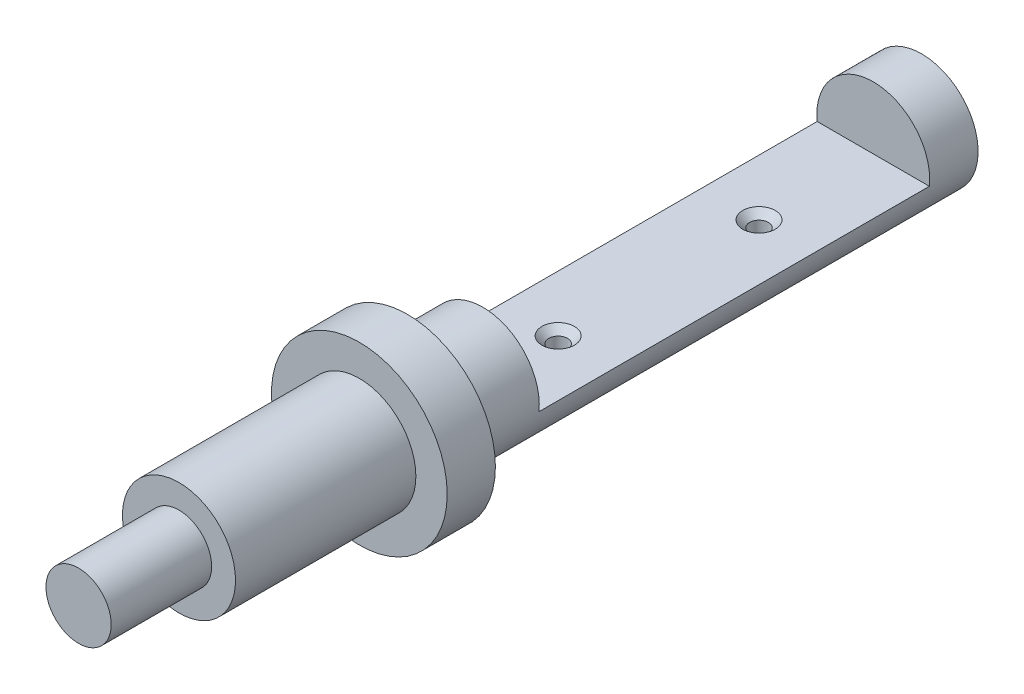
from build123d import *

# Parameters (mm, degrees)
SKETCH2_R                       = 7.1501
BOSS_EXTRUDE1_DEPTH             = 106.6292
SKETCH9_R                       = 11.1125
BOSS_EXTRUDE3_DEPTH             = 6.096
CUT_EXTRUDE1_DEPTH              = 49.3776
F_4_48_TAPPED_HOLE1_D           = 2.3749
F_4_48_TAPPED_HOLE1_CSINK_D     = 4.1148
F_4_48_TAPPED_HOLE1_CSINK_ANGLE = 90
SKETCH15_R                      = 7.1374
BOSS_EXTRUDE4_DEPTH             = 65.024
SKETCH16_OUTSIDE_W              = 46.46
SKETCH16_OUTSIDE_H              = 46.46
SKETCH16_OUTSIDE_R              = 7.1374
CUT_EXTRUDE2_DEPTH              = 65.024
CUT_EXTRUDE3_START              = 49.3776
CUT_EXTRUDE3_DEPTH              = 49.3776
SKETCH19_OUTSIDE_W              = 46.46
SKETCH19_OUTSIDE_H              = 46.46
SKETCH19_OUTSIDE_R              = 4.1275
CUT_EXTRUDE4_DEPTH              = 12.7
F_4_48_TAPPED_HOLE2_D           = 2.3749
F_4_48_TAPPED_HOLE2_CSINK_D     = 4.1148
F_4_48_TAPPED_HOLE2_CSINK_ANGLE = 90


with BuildPart() as part:
    # Sketch2 → Boss-Extrude1 (new body)
    with BuildSketch(Plane.XY):
        Circle(SKETCH2_R)
    extrude(amount=-BOSS_EXTRUDE1_DEPTH)

    # Sketch9 → Boss-Extrude3 (add)
    with BuildSketch(Plane.XY.offset(-35.5092)):
        Circle(SKETCH9_R)
    extrude(amount=-BOSS_EXTRUDE3_DEPTH)

    # Sketch11 → Cut-Extrude1 (cut)
    with BuildSketch(Plane(origin=(0, 0, -51.1302), x_dir=(-1, 0, 0), z_dir=(0, 0, -1))):
        with BuildLine():
            Line((-7.110729887, -0.7493), (7.110729887, -0.7493))
            ThreePointArc((7.110729887, -0.7493), (0, 7.1501), (-7.110729887, -0.7493))
        make_face()
    extrude(amount=CUT_EXTRUDE1_DEPTH, mode=Mode.SUBTRACT)

    # #4-48 Tapped Hole1 (through all)
    with Locations(Plane(origin=(0, -0.7493, 0), x_dir=(1, 0, 0), z_dir=(0, 1, 0))):
        with Locations((0, 86.0552), (0, 60.6552)):
            CounterSinkHole(F_4_48_TAPPED_HOLE1_D / 2, F_4_48_TAPPED_HOLE1_CSINK_D / 2, counter_sink_angle=F_4_48_TAPPED_HOLE1_CSINK_ANGLE)

    # Sketch15 → Boss-Extrude4 (add)
    with BuildSketch(Plane(origin=(0, 0, -106.6292), x_dir=(-1, 0, 0), z_dir=(0, 0, -1))):
        Circle(SKETCH15_R)
    extrude(amount=-BOSS_EXTRUDE4_DEPTH)

    # Sketch16 outside → Cut-Extrude2 (cut)
    with BuildSketch(Plane(origin=(0, 0, -106.6292), x_dir=(-1, 0, 0), z_dir=(0, 0, -1))):
        Rectangle(SKETCH16_OUTSIDE_W, SKETCH16_OUTSIDE_H)
        Circle(SKETCH16_OUTSIDE_R, mode=Mode.SUBTRACT)
    extrude(amount=-CUT_EXTRUDE2_DEPTH, mode=Mode.SUBTRACT)

    # Sketch18 → Cut-Extrude3 (cut)
    with BuildSketch(Plane(origin=(0, 0, -51.1302), x_dir=(-1, 0, 0), z_dir=(0, 0, -1)).offset(CUT_EXTRUDE3_START)):
        with BuildLine():
            Line((-7.096607271, -0.762), (7.096607271, -0.762))
            ThreePointArc((7.096607271, -0.762), (0, 7.1374), (-7.096607271, -0.762))
        make_face()
    extrude(amount=-CUT_EXTRUDE3_DEPTH, mode=Mode.SUBTRACT)

    # Sketch19 outside → Cut-Extrude4 (cut)
    with BuildSketch(Plane.XY):
        Rectangle(SKETCH19_OUTSIDE_W, SKETCH19_OUTSIDE_H)
        Circle(SKETCH19_OUTSIDE_R, mode=Mode.SUBTRACT)
    extrude(amount=-CUT_EXTRUDE4_DEPTH, mode=Mode.SUBTRACT)

    # #4-48 Tapped Hole2 (through all)
    with Locations(Plane(origin=(0, -0.762, 0), x_dir=(1, 0, 0), z_dir=(0, 1, 0))):
        with Locations((0, 60.6552), (0, 86.0552)):
            CounterSinkHole(F_4_48_TAPPED_HOLE2_D / 2, F_4_48_TAPPED_HOLE2_CSINK_D / 2, counter_sink_angle=F_4_48_TAPPED_HOLE2_CSINK_ANGLE)


solid = part.part
